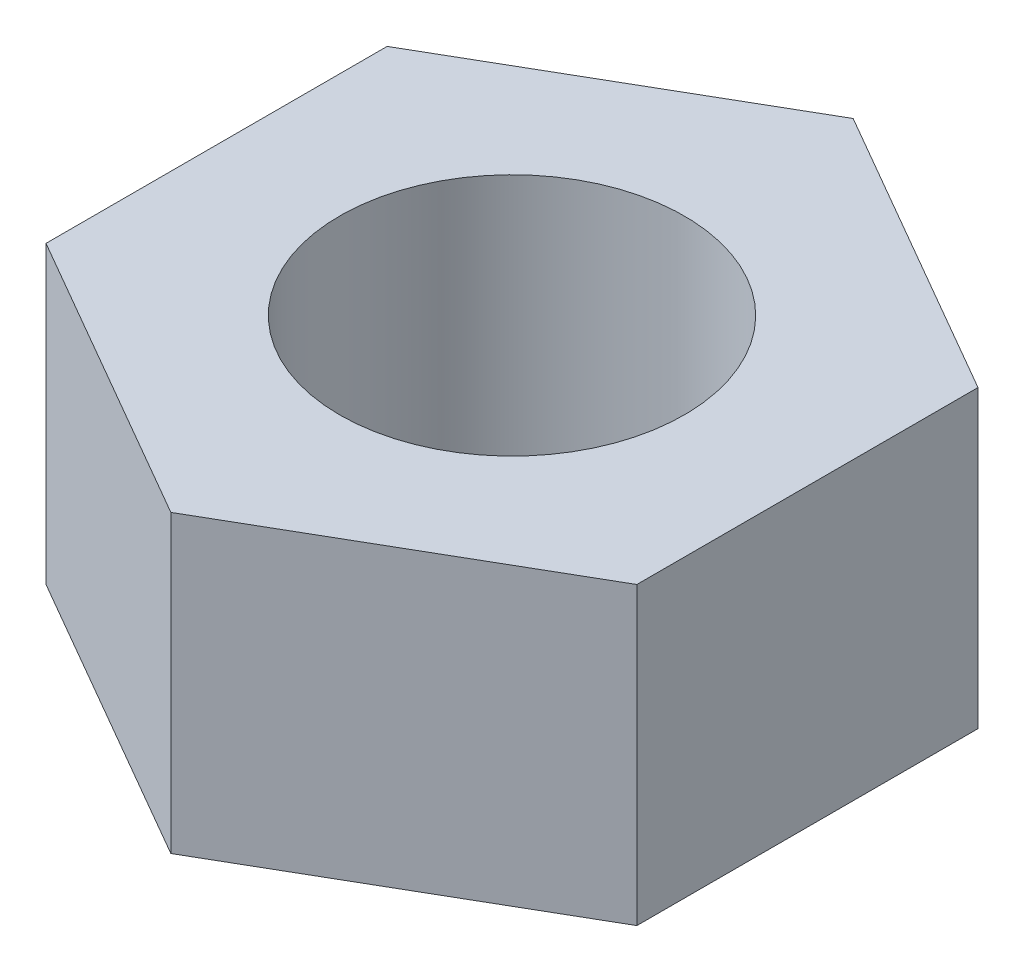
from build123d import *

# Parameters (mm, degrees)
EXTRUDE_1_DEPTH     = 15
HOLE_WIZARD_M20_1_D = 17.5


with BuildPart() as part:
    # 草图1 → 凸台-拉伸1 (new body)
    with BuildSketch(Plane(origin=(0, 0, 0), x_dir=(1, 0, 0), z_dir=(0, 1, 0))):
        Polygon((0, 17.320508076), (-15, 8.660254038), (-15, -8.660254038), (0, -17.320508076), (15, -8.660254038), (15, 8.660254038), align=None)
    extrude(amount=EXTRUDE_1_DEPTH)

    # M20 螺纹孔1 (through all)
    with Locations(Plane(origin=(0, 15, 0), x_dir=(1, 0, 0), z_dir=(0, 1, 0))):
        with Locations((0, 0)):
            Hole(HOLE_WIZARD_M20_1_D / 2)


solid = part.part
